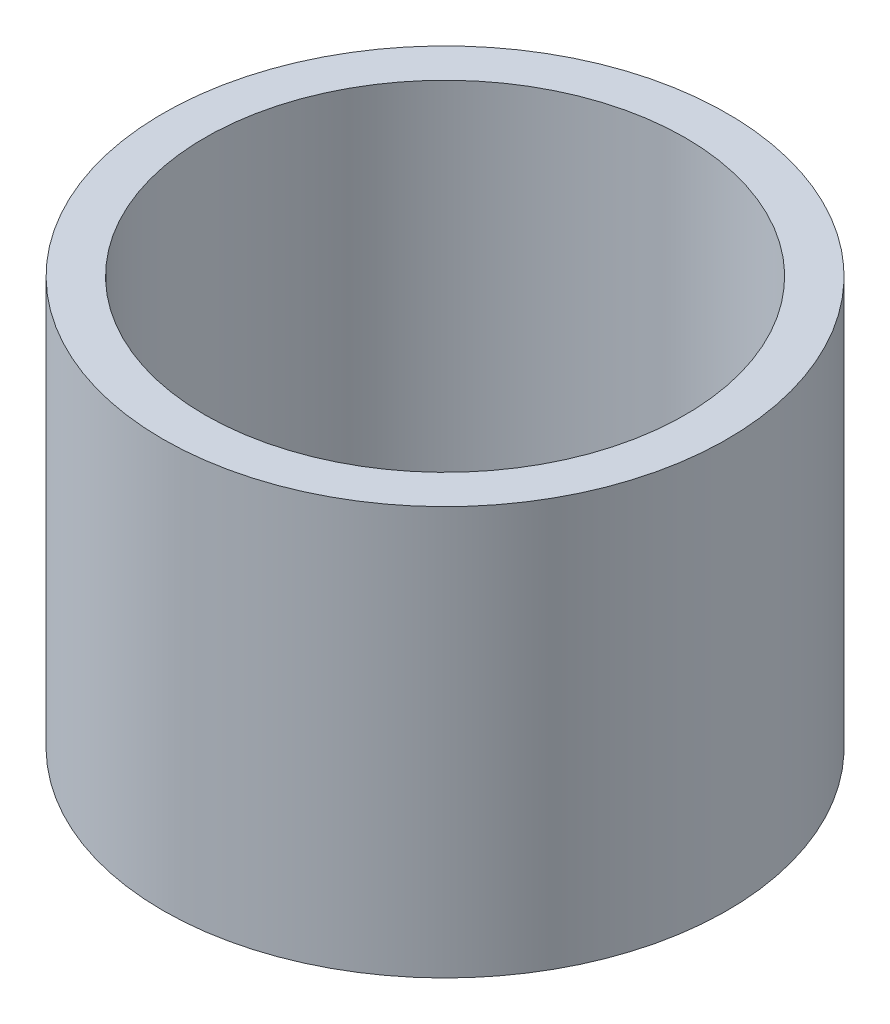
from build123d import *

# Parameters (mm, degrees)
SKETCH_1_R      = 23.5
SKETCH_1_R_2    = 20
EXTRUDE_1_DEPTH = 34


with BuildPart() as part:
    # 草图1 → 凸台-拉伸1 (new body)
    with BuildSketch(Plane(origin=(0, 0, 0), x_dir=(1, 0, 0), z_dir=(0, 1, 0))):
        with Locations(Location((0, 0, 0), (0, 0, 270))):
            Circle(SKETCH_1_R)
        with Locations(Location((0, 0, 0), (0, 0, 270))):
            Circle(SKETCH_1_R_2, mode=Mode.SUBTRACT)
    extrude(amount=EXTRUDE_1_DEPTH)


solid = part.part
